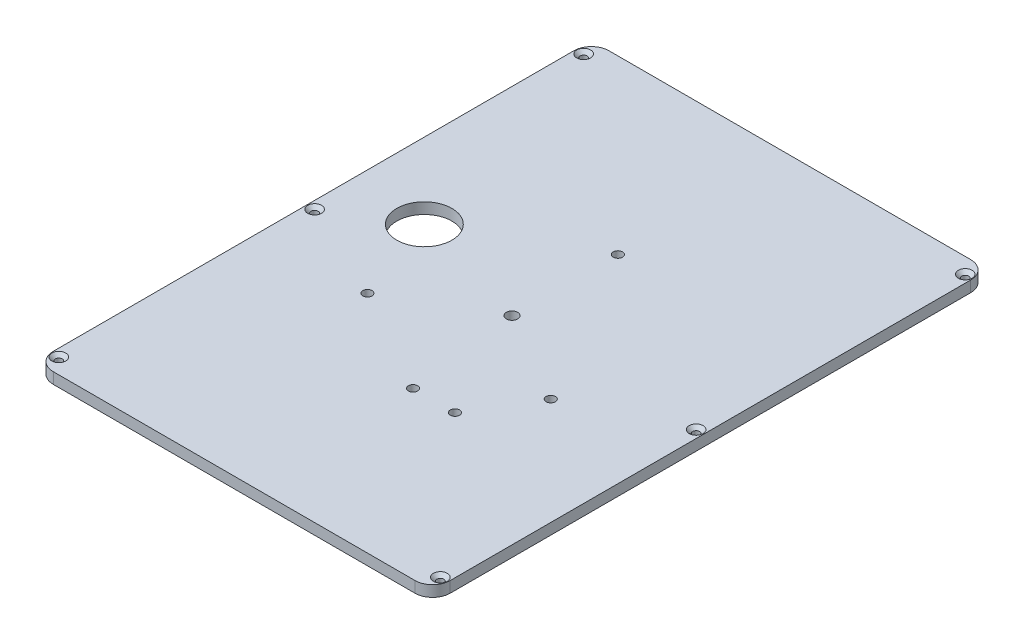
from build123d import *

# Parameters (mm, degrees)
SKETCH1_W                                       = 180
SKETCH1_H                                       = 252
BOSS_EXTRUDE1_DEPTH                             = 5
SKETCH2_R                                       = 70
BOSS_EXTRUDE2_DEPTH                             = 50
DOME1_FACE_RADIUS                               = 70
DOME1_HEIGHT                                    = 50
SKETCH3_R                                       = 2.1
CUT_EXTRUDE1_DEPTH                              = 188.085541932
CSK_FOR_M3_FLAT_HEAD_MACHINE_SCREW1_D           = 3.2
CSK_FOR_M3_FLAT_HEAD_MACHINE_SCREW1_DEPTH       = 8.5
CSK_FOR_M3_FLAT_HEAD_MACHINE_SCREW1_CSINK_D     = 6.3
CSK_FOR_M3_FLAT_HEAD_MACHINE_SCREW1_CSINK_ANGLE = 90
CSK_FOR_M3_FLAT_HEAD_MACHINE_SCREW1_TIP         = 0.96137699
SKETCH7_R                                       = 2.6
CUT_EXTRUDE3_DEPTH                              = 15
SKETCH9_W                                       = 180
SKETCH9_H                                       = 252
CUT_EXTRUDE4_DEPTH                              = 168
SKETCH11_R                                      = 12.5
CUT_EXTRUDE5_DEPTH                              = 49
FILLET1_R                                       = 8
M5_TAPPED_HOLE1_D                               = 4.2
M5_TAPPED_HOLE1_DEPTH                           = 14
M5_TAPPED_HOLE1_CSINK_D                         = 5.05
M5_TAPPED_HOLE1_CSINK_ANGLE                     = 90
M5_TAPPED_HOLE1_TIP                             = 1.2618073


with BuildPart() as part:
    # Sketch1 → Boss-Extrude1 (new body)
    with BuildSketch(Plane(origin=(0, 0, 0), x_dir=(1, 0, 0), z_dir=(0, 1, 0))):
        Rectangle(SKETCH1_W, SKETCH1_H)
    extrude(amount=BOSS_EXTRUDE1_DEPTH)

    # Sketch2 → Boss-Extrude2 (add)
    with BuildSketch(Plane(origin=(0, 5, 0), x_dir=(1, 0, 0), z_dir=(0, 1, 0))):
        with Locations(Location((0, 0, 0), (0, 0, 270))):
            Circle(SKETCH2_R)
    extrude(amount=BOSS_EXTRUDE2_DEPTH)

    # Dome1: a dome of height H over a round flat face of radius A is a cap of a sphere of radius (A * A + H * H) / (2 * H)
    dome1_r = (DOME1_FACE_RADIUS * DOME1_FACE_RADIUS + DOME1_HEIGHT * DOME1_HEIGHT) / (2 * DOME1_HEIGHT)
    dome1_base = Plane((0, 55, 0), z_dir=(0, 1, 0))
    with Locations(dome1_base.offset(DOME1_HEIGHT - dome1_r)):
        dome1_ball = Sphere(dome1_r, mode=Mode.PRIVATE)
    add(split(dome1_ball, bisect_by=dome1_base, keep=Keep.TOP, mode=Mode.PRIVATE))

    # Sketch3 → Cut-Extrude1 (cut, through all)
    with BuildSketch(Plane.XZ):
        with Locations(Location((0, -48, 0), (0, 0, 270))):
            Circle(SKETCH3_R)
        with Locations(Location((-41.569219382, 24, 0), (0, 0, 270))):
            Circle(SKETCH3_R)
        with Locations(Location((41.569219382, 24, 0), (0, 0, 270))):
            Circle(SKETCH3_R)
    extrude(amount=-CUT_EXTRUDE1_DEPTH, mode=Mode.SUBTRACT)

    # CSK for M3 Flat Head Machine Screw1
    with Locations(Plane(origin=(0, 5, 0), x_dir=(1, 0, 0), z_dir=(0, 1, 0))):
        with Locations((86.5, 119), (86.5, -3), (86.5, -119), (-86.5, -119), (-86.5, -3), (-86.5, 119)):
            CounterSinkHole(CSK_FOR_M3_FLAT_HEAD_MACHINE_SCREW1_D / 2, CSK_FOR_M3_FLAT_HEAD_MACHINE_SCREW1_CSINK_D / 2, depth=CSK_FOR_M3_FLAT_HEAD_MACHINE_SCREW1_DEPTH, counter_sink_angle=CSK_FOR_M3_FLAT_HEAD_MACHINE_SCREW1_CSINK_ANGLE)
            with Locations((0, 0, -(CSK_FOR_M3_FLAT_HEAD_MACHINE_SCREW1_DEPTH + CSK_FOR_M3_FLAT_HEAD_MACHINE_SCREW1_TIP / 2))):  # 118° drill point
                Cone(0, CSK_FOR_M3_FLAT_HEAD_MACHINE_SCREW1_D / 2, CSK_FOR_M3_FLAT_HEAD_MACHINE_SCREW1_TIP, mode=Mode.SUBTRACT)

    # Sketch7 → Cut-Extrude3 (cut)
    with BuildSketch(Plane.XZ):
        with Locations(Location((0, 0, 0), (0, 0, 270))):
            Circle(SKETCH7_R)
    extrude(amount=-CUT_EXTRUDE3_DEPTH, mode=Mode.SUBTRACT)

    # Sketch9 → Cut-Extrude4 (cut)
    with BuildSketch(Plane(origin=(0, 5, 0), x_dir=(1, 0, 0), z_dir=(0, 1, 0))):
        Rectangle(SKETCH9_W, SKETCH9_H)
    extrude(amount=CUT_EXTRUDE4_DEPTH, mode=Mode.SUBTRACT)

    # Sketch11 → Cut-Extrude5 (cut)
    with BuildSketch(Plane(origin=(0, 5, 0), x_dir=(1, 0, 0), z_dir=(0, 1, 0))):
        with Locations(Location((-55.749439459, 16, 0), (0, 0, 270))):
            Circle(SKETCH11_R)
    extrude(amount=-CUT_EXTRUDE5_DEPTH, mode=Mode.SUBTRACT)

    # Fillet1
    fillet1_edges = [part.edges().sort_by_distance(p)[0] for p in [
        (90, 2.5, 126),
        (-90, 2.5, 126),
        (-90, 2.5, -126),
        (90, 2.5, -126),
    ]]
    fillet(fillet1_edges, radius=FILLET1_R)

    # M5 Tapped Hole1
    with Locations(Plane(origin=(0, 0, 0), x_dir=(-1, 0, 0), z_dir=(0, -1, 0))):
        with Locations((-25.121103622, -51), (-6.121103622, -51)):
            CounterSinkHole(M5_TAPPED_HOLE1_D / 2, M5_TAPPED_HOLE1_CSINK_D / 2, depth=M5_TAPPED_HOLE1_DEPTH, counter_sink_angle=M5_TAPPED_HOLE1_CSINK_ANGLE)
            with Locations((0, 0, -(M5_TAPPED_HOLE1_DEPTH + M5_TAPPED_HOLE1_TIP / 2))):  # 118° drill point
                Cone(0, M5_TAPPED_HOLE1_D / 2, M5_TAPPED_HOLE1_TIP, mode=Mode.SUBTRACT)


solid = part.part
